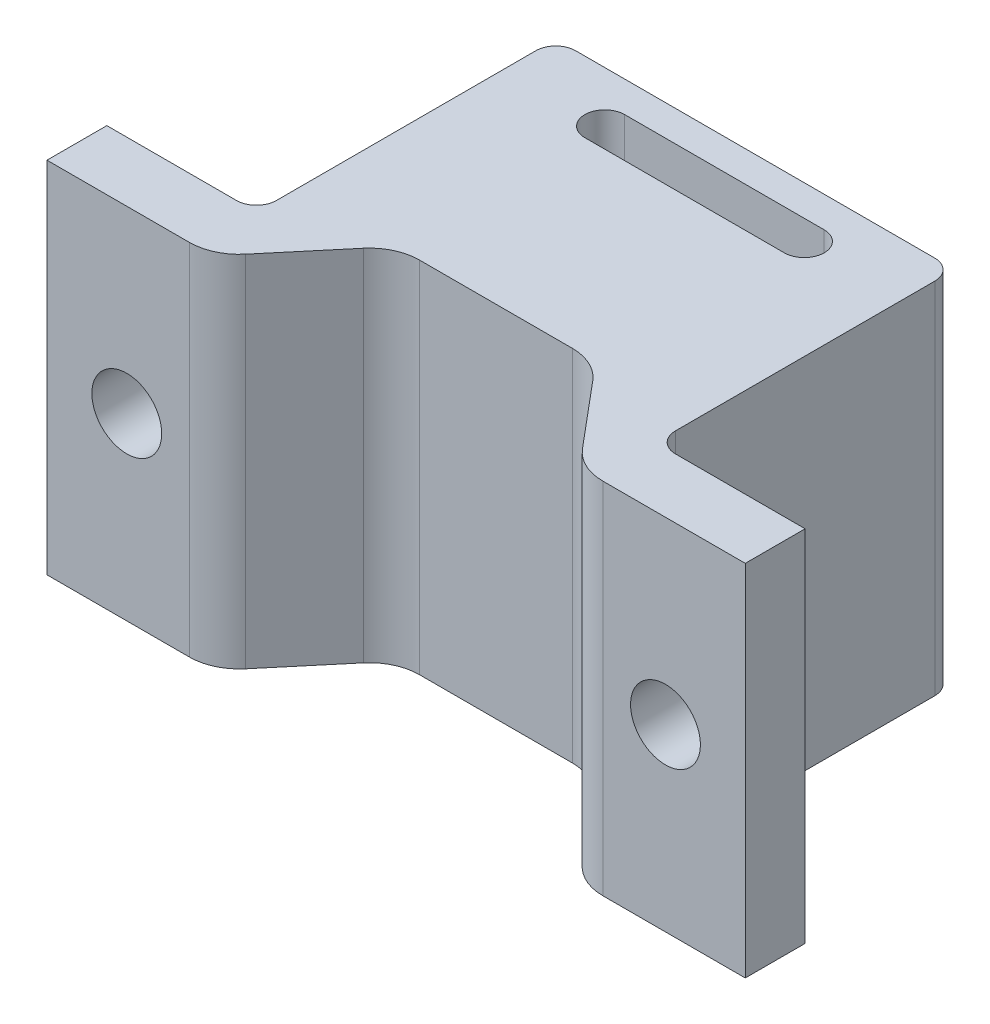
from build123d import *

# Parameters (mm, degrees)
BOSS_EXTRUDE1_DEPTH   = 36
FILLET1_R             = 5
FILLET2_R             = 2
SKETCH2_R             = 3.5
CUT_EXTRUDE1_DEPTH    = 59.489315264
SKETCH3_R             = 10
CUT_EXTRUDE2_DEPTH    = 6
SKETCH4_R             = 8
BOSS_EXTRUDE2_DEPTH   = 11.09
M8_TAPPED_HOLE1_D     = 6.8
M8_TAPPED_HOLE1_DEPTH = 22.25
M8_TAPPED_HOLE1_TIP   = 2.042926105
FILLET3_R             = 2


with BuildPart() as part:
    # Sketch1 → Boss-Extrude1 (new body)
    with BuildSketch(Plane(origin=(0, 0, 0), x_dir=(1, 0, 0), z_dir=(0, 1, 0))):
        Polygon((-20, -13.744612069), (-20, 16.255387931), (20, 16.255387931), (20, -13.744612069), (35, -13.744612069), (35, -19.744612069), (18.390996312, -19.744612069), (10, -9.744612069), (-10, -9.744612069), (-18.390996312, -19.744612069), (-35, -19.744612069), (-35, -13.744612069), align=None)
        with BuildLine():
            Line((-10, 13.167446825), (10, 13.167446825))
            ThreePointArc((10, 13.167446825), (12, 11.167446825), (10, 9.167446825))
            Line((10, 9.167446825), (-10, 9.167446825))
            ThreePointArc((-10, 9.167446825), (-12, 11.167446825), (-10, 13.167446825))
        make_face(mode=Mode.SUBTRACT)
    extrude(amount=BOSS_EXTRUDE1_DEPTH)

    # Fillet1
    fillet1_edges = [part.edges().sort_by_distance(p)[0] for p in [
        (18.390996312, 18, 19.744612069),
        (10, 18, 9.744612069),
        (-10, 18, 9.744612069),
        (-18.390996312, 18, 19.744612069),
    ]]
    fillet(fillet1_edges, radius=FILLET1_R)

    # Fillet2
    fillet2_edges = [part.edges().sort_by_distance(p)[0] for p in [
        (20, 18, 13.744612069),
        (-20, 18, 13.744612069),
    ]]
    fillet(fillet2_edges, radius=FILLET2_R)

    # Sketch2 → Cut-Extrude1 (cut, through all)
    with BuildSketch(Plane(origin=(0, 0, 13.744612069), x_dir=(-1, 0, 0), z_dir=(0, 0, -1))):
        with Locations((-27, 18)):
            Circle(SKETCH2_R)
        with Locations((27, 18)):
            Circle(SKETCH2_R)
    extrude(amount=-CUT_EXTRUDE1_DEPTH, mode=Mode.SUBTRACT)

    # Sketch3 → Cut-Extrude2 (cut)
    with BuildSketch(Plane(origin=(0, 0, -16.255387931), x_dir=(-1, 0, 0), z_dir=(0, 0, -1))):
        with Locations((0, 18)):
            Circle(SKETCH3_R)
    extrude(amount=-CUT_EXTRUDE2_DEPTH, mode=Mode.SUBTRACT)

    # Sketch4 → Boss-Extrude2 (add)
    with BuildSketch(Plane(origin=(0, 0, -9.167446825), x_dir=(-1, 0, 0), z_dir=(0, 0, -1))):
        with Locations((0, 18)):
            Circle(SKETCH4_R)
    extrude(amount=BOSS_EXTRUDE2_DEPTH)

    # M8 Tapped Hole1
    with Locations(Plane(origin=(0, 0, -20.257446825), x_dir=(-1, 0, 0), z_dir=(0, 0, -1))):
        with Locations((0, 18)):
            Hole(M8_TAPPED_HOLE1_D / 2, depth=M8_TAPPED_HOLE1_DEPTH)
            with Locations((0, 0, -(M8_TAPPED_HOLE1_DEPTH + M8_TAPPED_HOLE1_TIP / 2))):  # 118° drill point
                Cone(0, M8_TAPPED_HOLE1_D / 2, M8_TAPPED_HOLE1_TIP, mode=Mode.SUBTRACT)

    # Fillet3
    fillet3_edges = [part.edges().sort_by_distance(p)[0] for p in [
        (-20, 18, -16.255387931),
        (20, 18, -16.255387931),
    ]]
    fillet(fillet3_edges, radius=FILLET3_R)


solid = part.part
